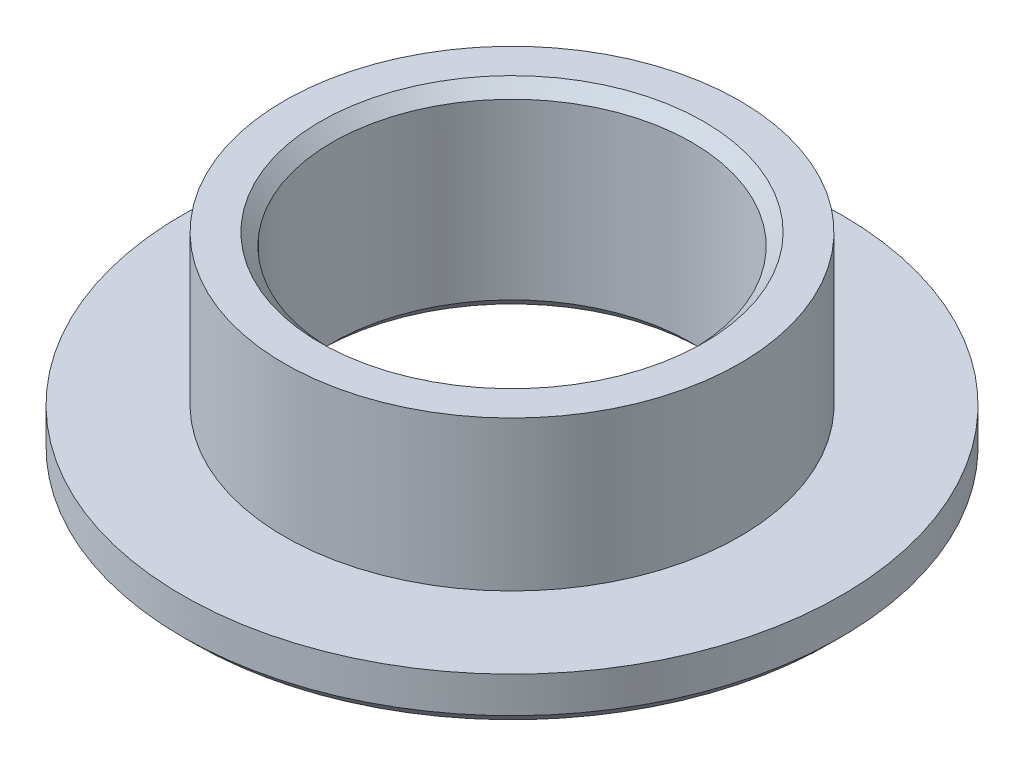
from build123d import *

# Parameters (mm, degrees)
CHAMFER1_SIZE = 2


with BuildPart() as part:
    # Sketch1 → Revolve1 (revolve)
    with BuildSketch(Plane.XY, mode=Mode.PRIVATE) as revolve1_sk:
        Polygon((-30, 0), (-30, 33), (-38, 33), (-38, 8), (-55, 8), (-55, 0), align=None)
    revolve(revolve1_sk.sketch.rotate(Axis((0, 0, 0), (0, 1, 0)), 270), axis=Axis((0, 0, 0), (0, 1, 0)))

    # Chamfer1
    chamfer1_edges = [part.edges().sort_by_distance(p)[0] for p in [
        (0, 0, 55),
        (0, 33, 30),
        (0, 0, 30),
    ]]
    chamfer(chamfer1_edges, length=CHAMFER1_SIZE)


solid = part.part
